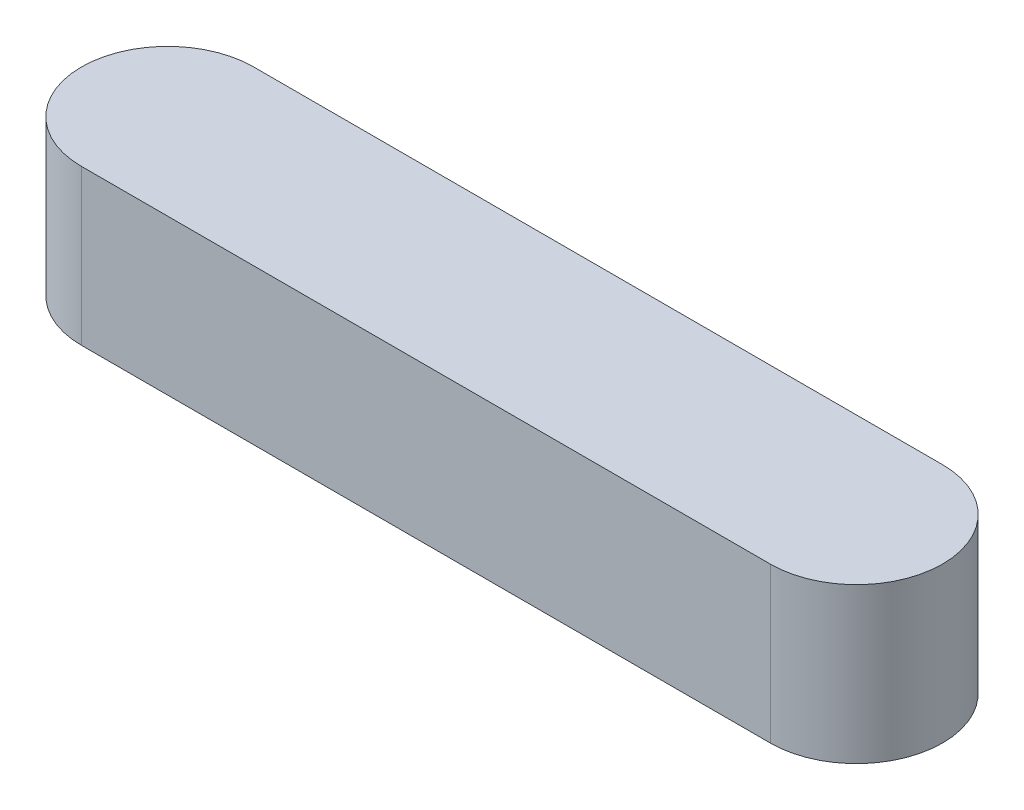
SolidWorks part; units mm, degrees
ref_plane "Front Plane" through (0, 0, 0) normal (0, 0, 1) x (1, 0, 0)
ref_plane "Top Plane" through (0, 0, 0) normal (0, 1, 0) x (1, 0, 0)
ref_plane "Right Plane" through (0, 0, 0) normal (1, 0, 0) x (0, 0, -1)
sketch "Sketch1" plane through (0, 0, 0) normal (0, 1, 0) x (1, 0, 0)
  line L0 (-75.6521, 0) -> (65.3269, 0) construction
  line L1 (-10, 2.5) -> (10, 2.5)
  line L2 (10, -2.5) -> (-10, -2.5)
  line L3 (0, 9.5065) -> (0, -7.1206) construction
  arc A0 (10, 2.5) -> (10, -2.5) centre (10, 0) cw
  arc A1 (-10, -2.5) -> (-10, 2.5) centre (-10, 0) cw
  dimension "D1" = 5
  dimension "D2" = 20
extrude "Boss-Extrude1" add sketch "Sketch1" along normal blind 4.5
